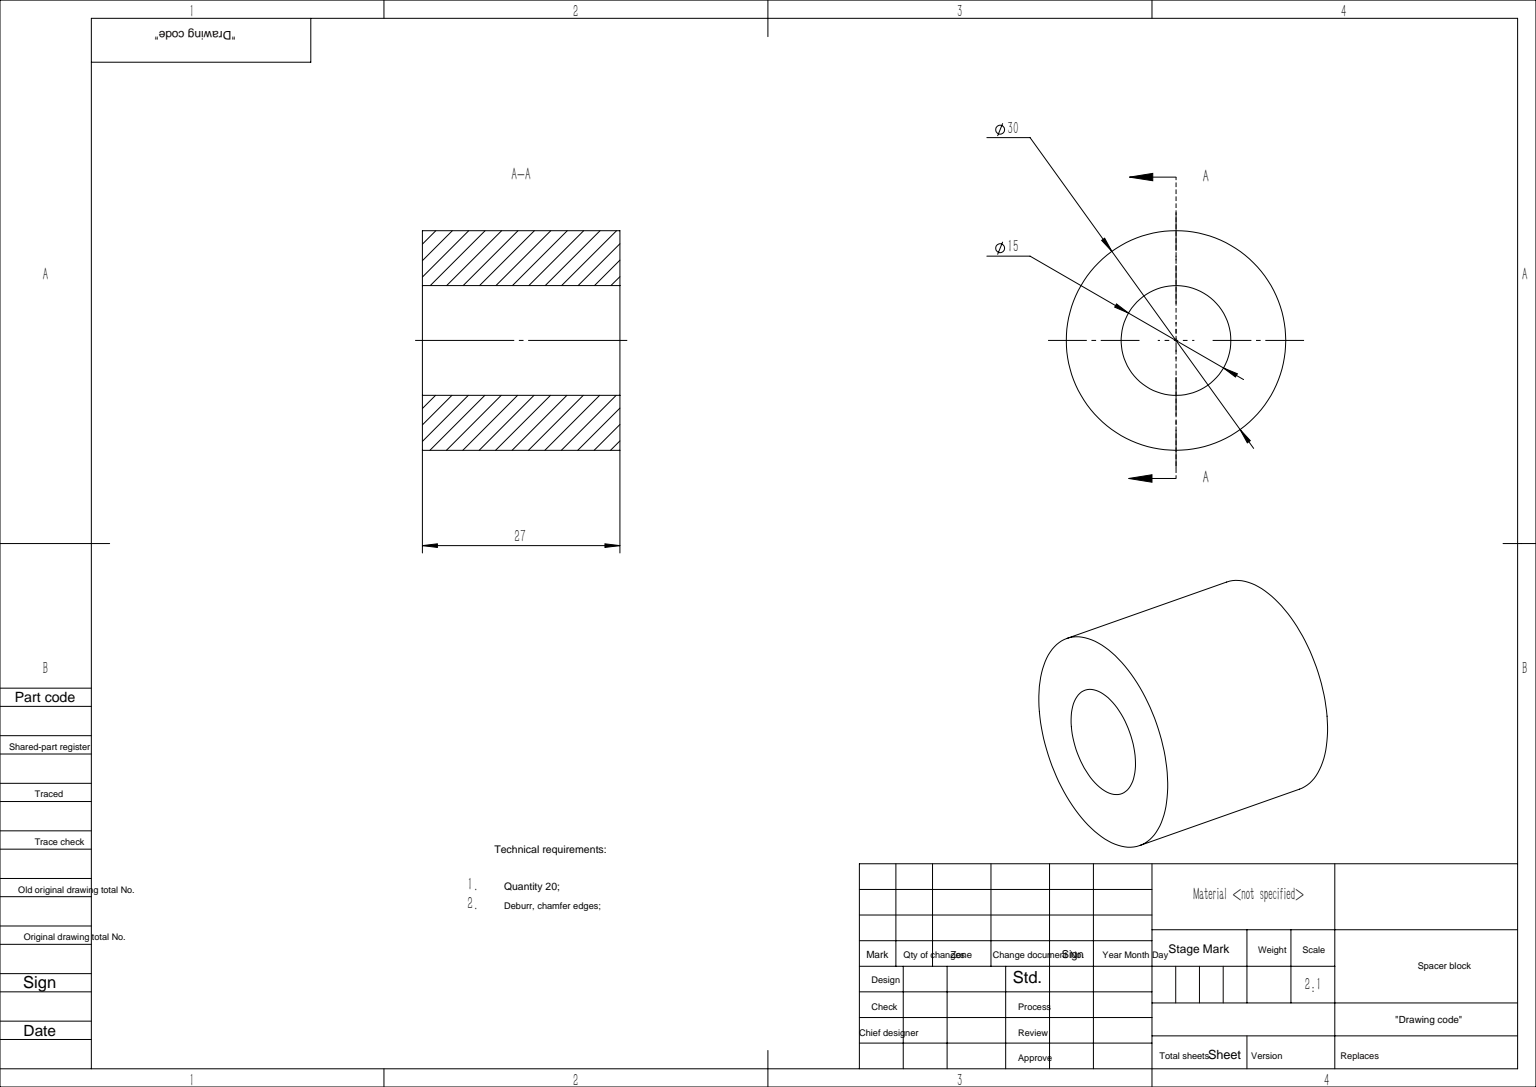
SolidWorks part; units mm, degrees
ref_plane "前视基准面" through (0, 0, 0) normal (0, 0, 1) x (1, 0, 0)
ref_plane "上视基准面" through (0, 0, 0) normal (0, 1, 0) x (1, 0, 0)
ref_plane "右视基准面" through (0, 0, 0) normal (1, 0, 0) x (0, 0, -1)
sketch "草图1" plane through (0, 0, -471) normal (0, 0, -1) x (-1, 0, 0)
  circle A0 centre (-645.9391, 1570.019) radius 7.5 construction
  circle A1 centre (-645.9391, 1570.019) radius 7.5
  circle A2 centre (-645.9391, 1570.019) radius 15
  dimension "D1" = 30
extrude "凸台-拉伸1" add sketch "草图1" along normal up to surface (27 mm away)
